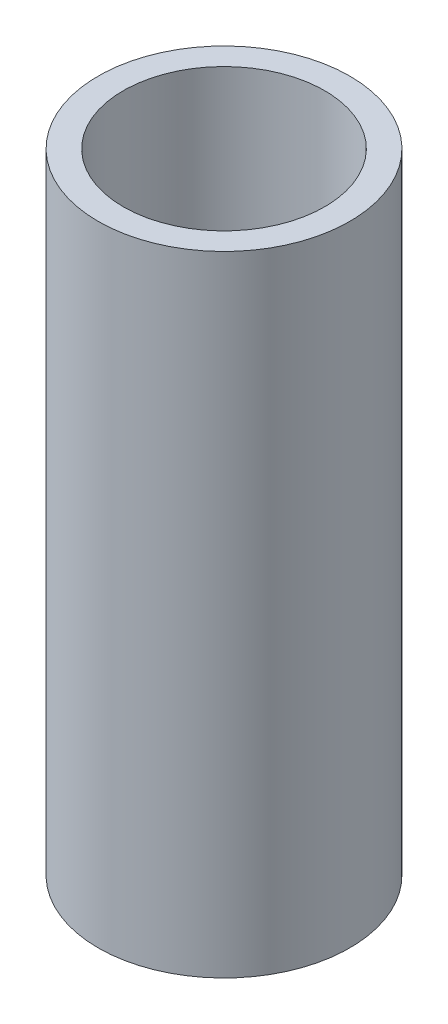
from build123d import *

# Parameters (mm, degrees)
SKETCH1_R           = 10
SKETCH1_R_2         = 8
BOSS_EXTRUDE1_DEPTH = 50


with BuildPart() as part:
    # Sketch1 → Boss-Extrude1 (new body)
    with BuildSketch(Plane(origin=(0, 0, 0), x_dir=(1, 0, 0), z_dir=(0, 1, 0))):
        with Locations(Location((0, 0, 0), (0, 0, 270))):
            Circle(SKETCH1_R)
        with Locations(Location((0, 0, 0), (0, 0, 270))):
            Circle(SKETCH1_R_2, mode=Mode.SUBTRACT)
    extrude(amount=BOSS_EXTRUDE1_DEPTH)


solid = part.part
